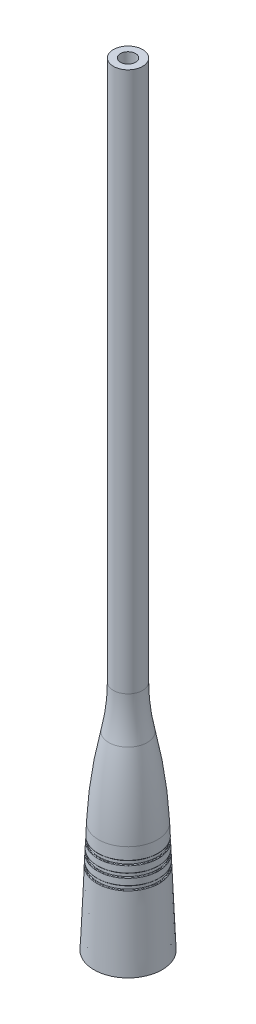
from build123d import *

# Parameters (mm, degrees)
FILLET_3_R = 0.1


with BuildPart() as part:
    # 草图1 → 旋转1 (revolve)
    with BuildSketch(Plane.XY, mode=Mode.PRIVATE) as revolve_1_sk:
        with BuildLine():
            Line((-7.4, 0), (-6.733333333, 16))
            Line((-6.733333333, 16), (-6.483116414, 16))
            Line((-6.483116414, 16), (-6.44978308, 16.8))
            Line((-6.44978308, 16.8), (-6.7, 16.8))
            Line((-6.7, 16.8), (-6.6375, 18.3))
            Line((-6.6375, 18.3), (-6.38728308, 18.3))
            Line((-6.38728308, 18.3), (-6.353949747, 19.1))
            Line((-6.353949747, 19.1), (-6.604166667, 19.1))
            Line((-6.604166667, 19.1), (-6.541666667, 20.6))
            Line((-6.541666667, 20.6), (-6.291449747, 20.6))
            Line((-6.291449747, 20.6), (-6.258116414, 21.4))
            Line((-6.258116414, 21.4), (-6.508333333, 21.4))
            Line((-6.508333333, 21.4), (-6.4, 24))
            ThreePointArc((-6.4, 24), (-5.663407353, 32.642384563), (-4.180674763, 41.18842948))
            ThreePointArc((-4.180674763, 41.18842948), (-3.427147619, 45.817139569), (-3.175, 50.5))
            Line((-3.175, 50.5), (-3.175, 168))
            Line((-3.175, 168), (-1.65, 168))
            Line((-1.65, 168), (-1.65, 40))
            Line((-1.65, 40), (-3.75, 40))
            Line((-3.75, 40), (-3.75, 10.5))
            Line((-3.75, 10.5), (-4.75, 10.5))
            Line((-4.75, 10.5), (-4.75, 2.5))
            Line((-4.75, 2.5), (-6.2, 2.5))
            Line((-6.2, 2.5), (-6.2, 0))
            Line((-6.2, 0), (-7.4, 0))
        make_face()
    revolve(revolve_1_sk.sketch.rotate(Axis((0, 0, 0), (0, 1, 0)), 270), axis=Axis((0, 0, 0), (0, 1, 0)))

    # 圆角3
    fillet_3_edges = [part.edges().sort_by_distance(p)[0] for p in [
        (0, 16, 6.733333333),
        (0, 16, 6.483116414),
        (0, 16.8, 6.44978308),
        (0, 16.8, 6.7),
        (0, 18.3, 6.6375),
        (0, 18.3, 6.38728308),
        (0, 19.1, 6.353949747),
        (0, 19.1, 6.604166667),
        (0, 20.6, 6.541666667),
        (0, 20.6, 6.291449747),
        (0, 21.4, 6.258116414),
        (0, 21.4, 6.508333333),
    ]]
    fillet(fillet_3_edges, radius=FILLET_3_R)


solid = part.part
